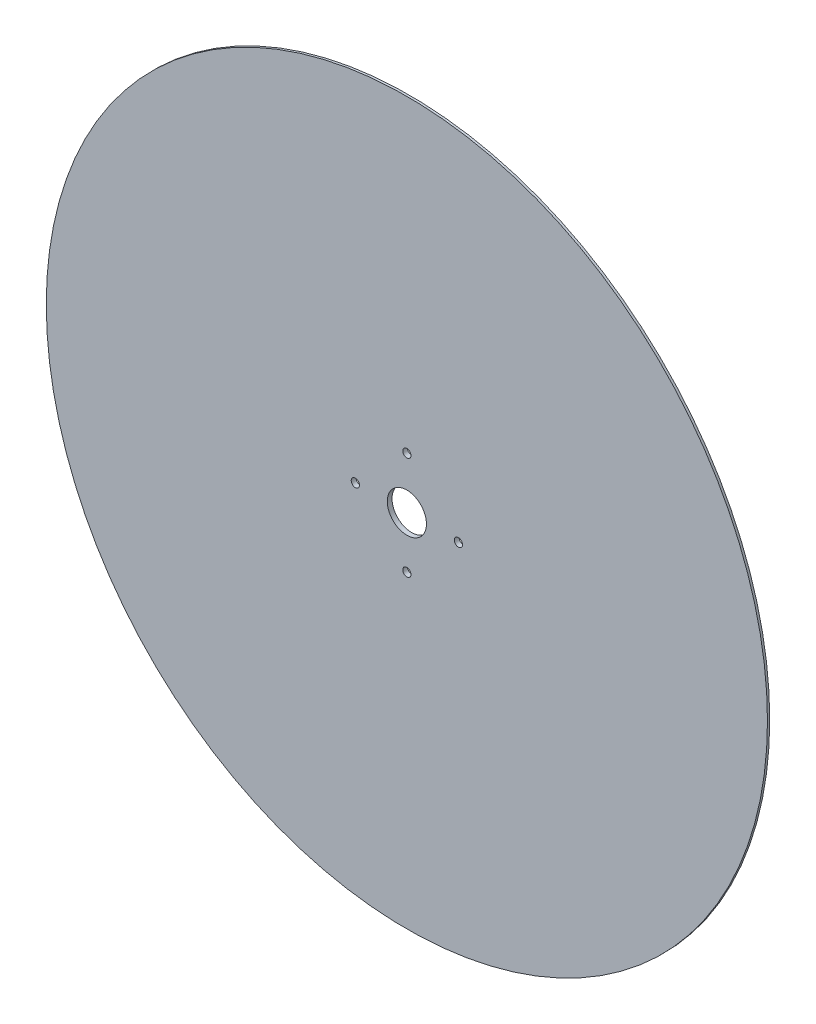
SolidWorks part; units mm, degrees
ref_plane "前视基准面" through (0, 0, 0) normal (0, 0, 1) x (1, 0, 0)
ref_plane "上视基准面" through (0, 0, 0) normal (0, 1, 0) x (1, 0, 0)
ref_plane "右视基准面" through (0, 0, 0) normal (1, 0, 0) x (0, 0, -1)
sketch "草图3" plane through (0, 0, 0) normal (0, 0, 1) x (1, 0, 0)
  circle A0 centre (0, 0) radius 175
  dimension "D1" = 350
extrude "凸台-拉伸1" add sketch "草图3" along normal blind 1.1
sketch "草图4" plane through (0, 0, 0) normal (0, 0, -1) x (-1, 0, 0)
  circle A0 centre (0, 0) radius 170
  dimension "D1" = 340
extrude "凸台-拉伸2" add sketch "草图4" along normal blind 1.2
sketch "草图7" plane through (0, 0, 1.1) normal (0, 0, 1) x (1, 0, 0)
  circle A0 centre (0, 0) radius 9.5
  dimension "D1" = 19
extrude "切除-拉伸1" cut sketch "草图7" against normal through all
sketch "草图8" plane through (0, 0, 0) normal (0, 1, 0) x (1, 0, 0)
  line L0 (-175, 0) -> (-170, 1.2)
  line L1 (-170, 1.2) -> (-170, 0)
  line L2 (-170, 0) -> (-175, 0)
sketch "草图9" plane through (0, 0, 0) normal (0, 0, -1) x (-1, 0, 0)
  circle A0 centre (0, 0) radius 170
  dimension "D1" = 340
sweep "扫描1" add profiles "草图8" path "草图9"
sketch "草图10" plane through (0, 0, 1.1) normal (0, 0, 1) x (1, 0, 0)
  circle A0 centre (0, 0) radius 25 construction
  circle A1 centre (0, 25) radius 2
  circle A2 centre (25, 0) radius 2
  circle A3 centre (0, -25) radius 2
  circle A4 centre (-25, 0) radius 2
  dimension "D1" = 50
  dimension "D2" = 4
extrude "切除-拉伸2" cut sketch "草图10" against normal up to surface (2.3 mm away) up to face at (9.5, 0, -1.2)
